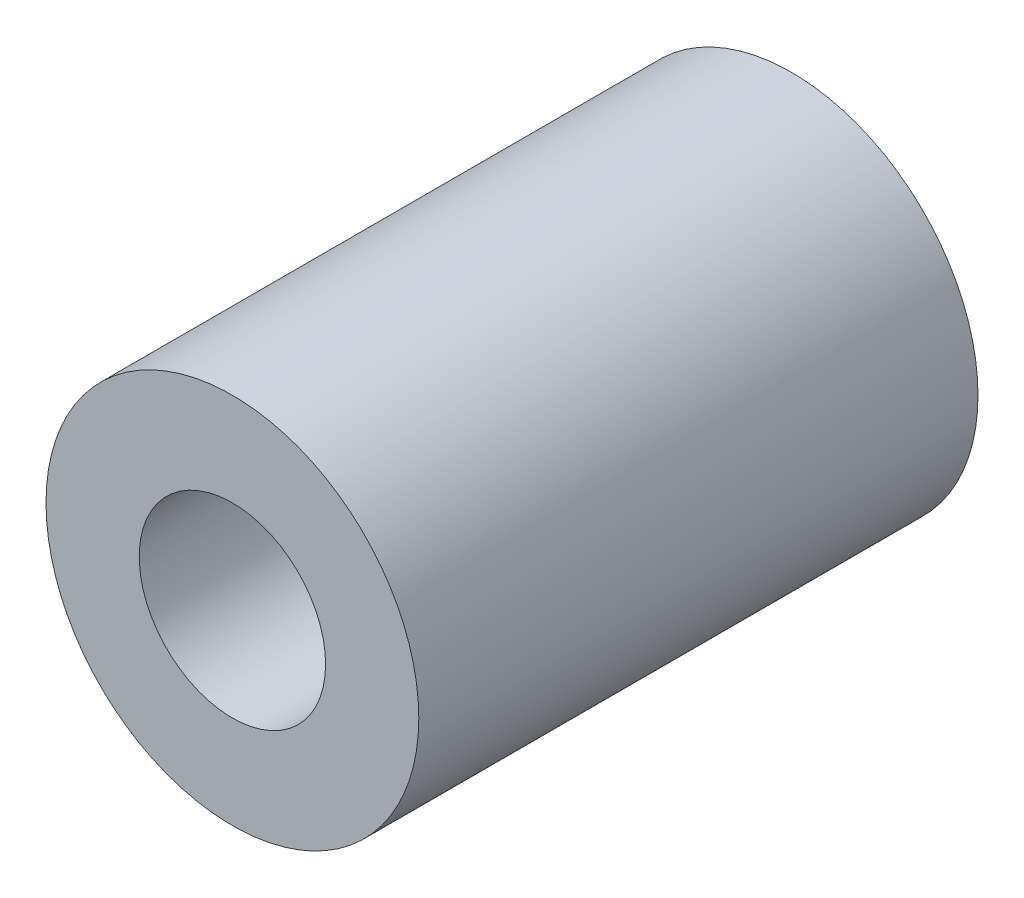
from build123d import *

# Parameters (mm, degrees)
SKETCH_1_R      = 8
SKETCH_1_R_2    = 4
EXTRUDE_1_DEPTH = 12


with BuildPart() as part:
    # 草图1 → 凸台-拉伸1 (new, symmetric)
    with BuildSketch(Plane.XY):
        Circle(SKETCH_1_R)
        Circle(SKETCH_1_R_2, mode=Mode.SUBTRACT)
    extrude(amount=EXTRUDE_1_DEPTH, both=True)


solid = part.part
